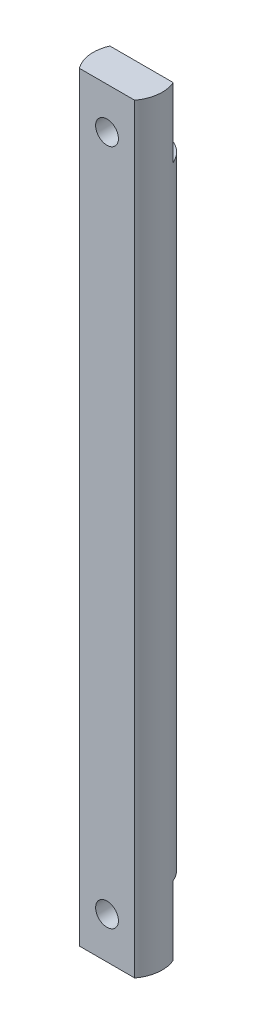
from build123d import *

# Parameters (mm, degrees)
SKETCH1_R           = 5
BOSS_EXTRUDE1_DEPTH = 110
CUT_EXTRUDE1_DEPTH  = 111.227038425
CUT_EXTRUDE2_START  = -10
CUT_EXTRUDE2_DEPTH  = 10
M4_TAPPED_HOLE2_D   = 3.3


with BuildPart() as part:
    # Sketch1 → Boss-Extrude1 (new body)
    with BuildSketch(Plane(origin=(0, 0, 0), x_dir=(1, 0, 0), z_dir=(0, 1, 0))):
        with Locations(Location((0, 0, 0), (0, 0, 270))):
            Circle(SKETCH1_R)
    extrude(amount=BOSS_EXTRUDE1_DEPTH)

    # Sketch2 → Cut-Extrude1 (cut, through all)
    with BuildSketch(Plane(origin=(0, 110, 0), x_dir=(1, 0, 0), z_dir=(0, 1, 0))):
        with BuildLine():
            Line((-4, -3), (4, -3))
            ThreePointArc((4, -3), (0, -5), (-4, -3))
        make_face()
    extrude(amount=-CUT_EXTRUDE1_DEPTH, mode=Mode.SUBTRACT)

    # Sketch3 → Cut-Extrude2 (cut)
    with BuildSketch(Plane(origin=(0, 110, 0), x_dir=(1, 0, 0), z_dir=(0, 1, 0)).offset(CUT_EXTRUDE2_START)):
        with BuildLine():
            Line((-4.582575695, 2), (4.582575695, 2))
            ThreePointArc((4.582575695, 2), (0, 5), (-4.582575695, 2))
        make_face()
    cut_extrude2 = extrude(amount=CUT_EXTRUDE2_DEPTH, mode=Mode.SUBTRACT)

    # Mirror1: Cut-Extrude2 across plane
    add(cut_extrude2.mirror(Plane.ZX.offset(55)), mode=Mode.SUBTRACT)

    # M4 Tapped Hole2 (through all)
    with Locations(Plane(origin=(0, 0, -2), x_dir=(-1, 0, 0), z_dir=(0, 0, -1))):
        with Locations((0, 104), (0, 6)):
            Hole(M4_TAPPED_HOLE2_D / 2)


solid = part.part
